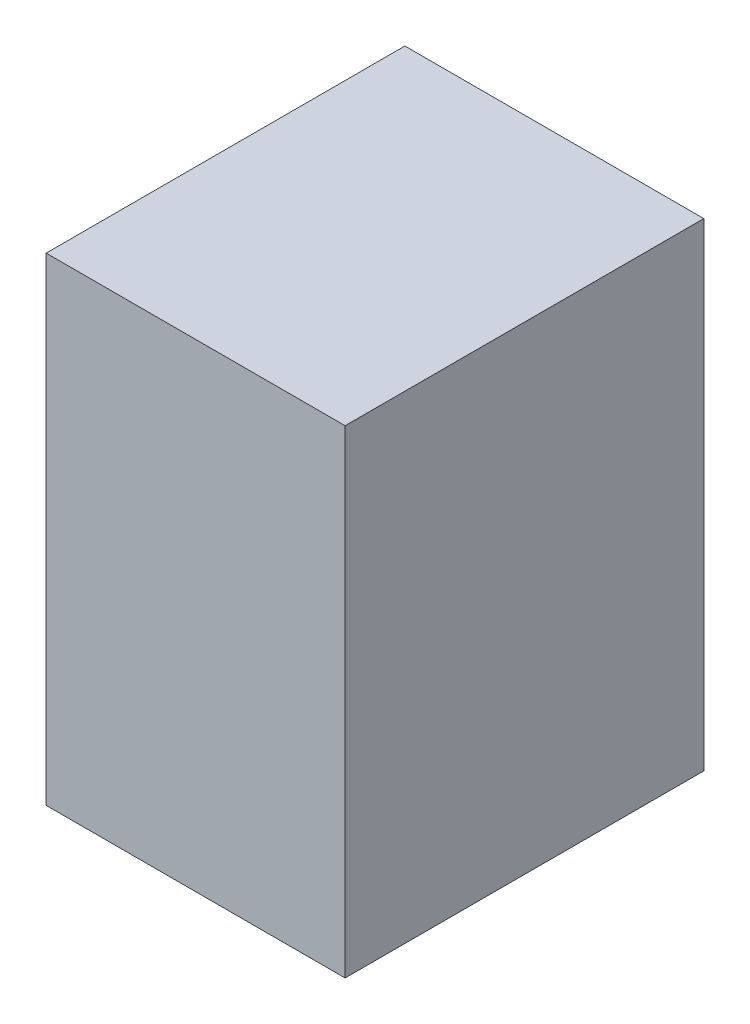
from build123d import *

# Parameters (mm, degrees)
SKETCH1_W           = 250
SKETCH1_H           = 400
BOSS_EXTRUDE1_DEPTH = 300


with BuildPart() as part:
    # Sketch1 → Boss-Extrude1 (new body)
    with BuildSketch(Plane.XY):
        Rectangle(SKETCH1_W, SKETCH1_H)
    extrude(amount=BOSS_EXTRUDE1_DEPTH)


solid = part.part
